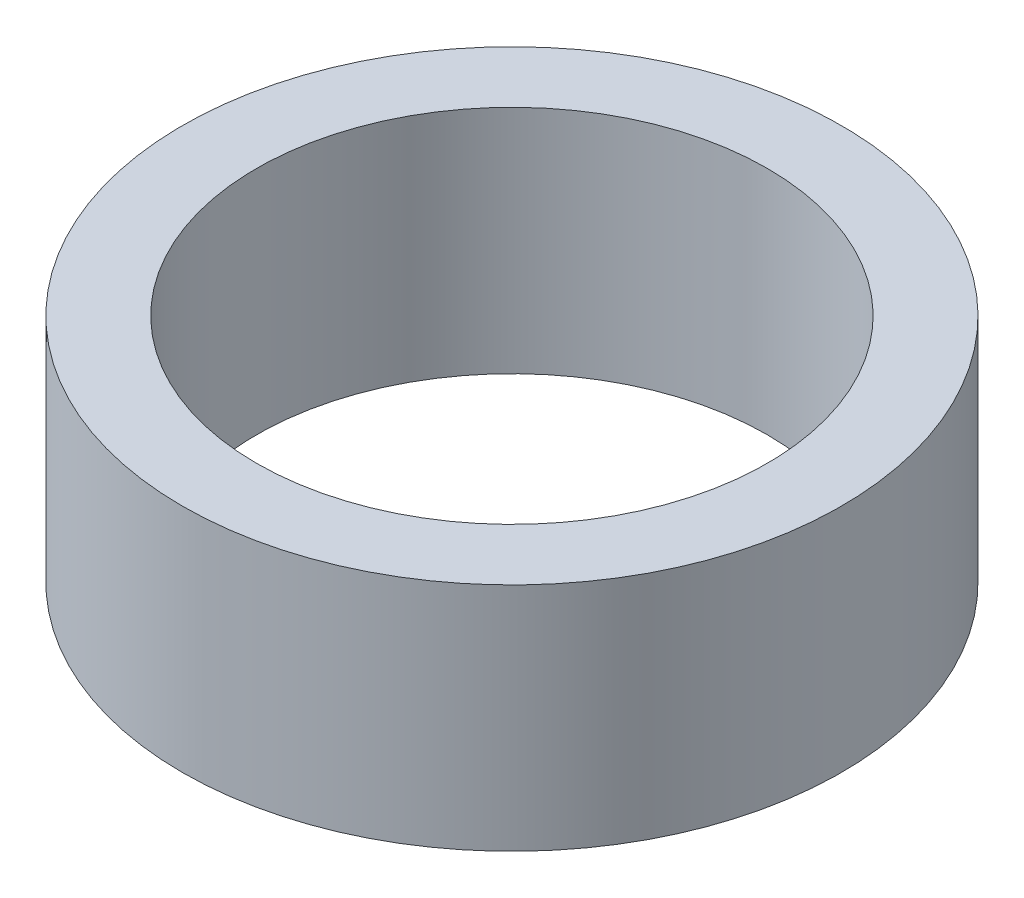
SolidWorks part; units mm, degrees
ref_plane "Front Plane" through (0, 0, 0) normal (0, 0, 1) x (1, 0, 0)
ref_plane "Top Plane" through (0, 0, 0) normal (0, 1, 0) x (1, 0, 0)
ref_plane "Right Plane" through (0, 0, 0) normal (1, 0, 0) x (0, 0, -1)
sketch "Sketch1" plane through (0, 0, 0) normal (0, 1, 0) x (1, 0, 0)
  circle A0 centre (0, 0) radius 4
  circle A1 centre (0, 0) radius 3.1
  dimension "D1" = 6.2
  dimension "D2" = 8
extrude "Boss-Extrude1" add sketch "Sketch1" along normal blind 2.8
